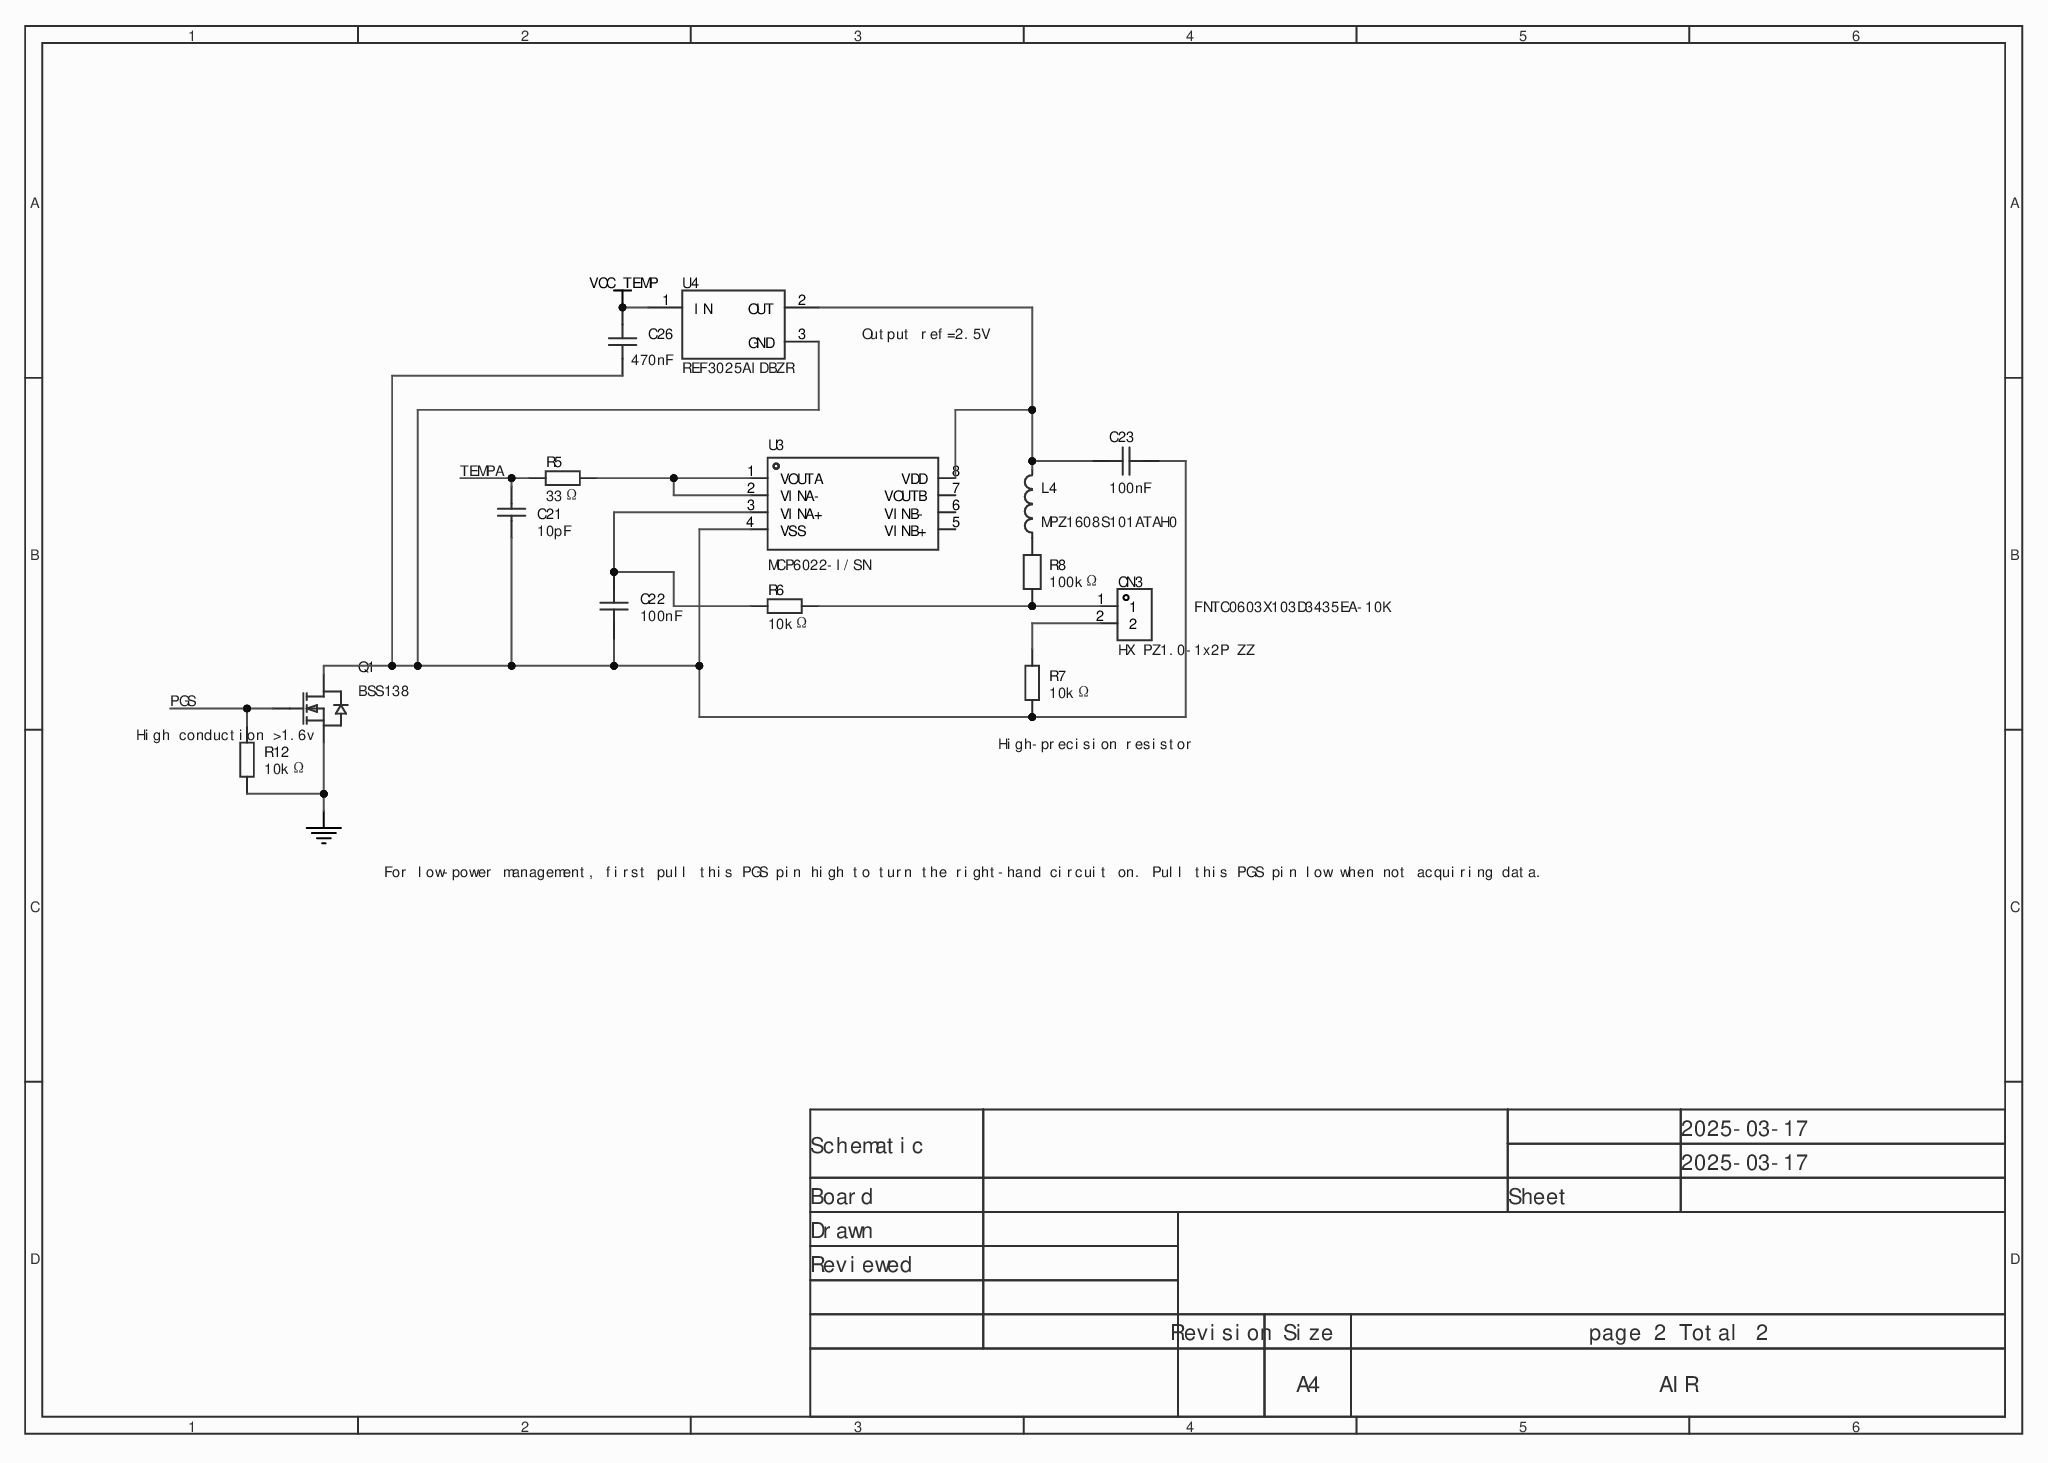
[diagram p0: MISC82703-4.schdoc]
# Altium project MISC82703-11.PrjPCB
2 sheets, 42 parts. Net scope: global (net labels, ports and power ports of the same name join across sheets).
Board file: MISC82703.PcbDoc
Sheets:
  MISC82703-4.schdoc
  MISC82703-2.schdoc

## Sheet MISC82703-4.schdoc
size 307 x 218 mm; Version: V1.0; @Project Name: MISC82703; @Page Count: 2; @Update Date: 2025-03-17; @Create Date: 2025-03-17; @Schematic Name: MISC82703; @Page No: 2; @Create Time: 21:29:07; @Update Time: 21:29:09; @Board Name: MISC82703

### Parts
C21  10pF  [C0402]
C22  100nF  [C0402]
C23  100nF  [C0402]
C26  470nF  [C0402]
CN3  HX PZ1.0-1x2P ZZ  [HDR-TH_2P-P1.00-V-M]
L4  MPZ1608S101ATAH0  [L0603]
Q1  BSS138  [SOT-23-3_L3.0-W1.7-P0.95-LS2.9-BR]
R5  33Ω  [R0402]
R6  10kΩ  [R0402]
R7  10kΩ  [R0402]
R8  100kΩ  [R0402]
R12  10kΩ  [R0402]
U3  MCP6022-I/SN  [SOIC-8_L4.9-W3.9-P1.27-LS6.0-BL]
U4  REF3025AIDBZR  [SOT-23-3_L2.9-W1.6-P1.90-LS2.8-BR]

### Nets
GND: Q1.2(S) R12.1
VCC_TEMP: C26.2 U4.1(IN)  [project net TL_VDD3]
PGS: Q1.1(G) R12.2
TEMPA: C21.2 R5.1
NetC21_1: C21.1 C22.1 C23.2 C26.1 Q1.3(D) R7.1 U3.4(VSS) U4.3(GND)
NetC22_2: C22.2 R6.2 U3.3(VINA+)
NetC23_1: C23.1 L4.2 U3.8(VDD) U4.2(OUT)
NetCN3_1: CN3.1 R6.1 R8.1
NetCN3_2: CN3.2 R7.2
NetL4_1: L4.1 R8.2
NetR5_2: R5.2 U3.1(VOUTA) U3.2(VINA-)

Not connected (* = marked no-connect by the designer): U3 5(VINB+)* 6(VINB-)* 7(VOUTB)*

### Notes on the sheet
- Output ref=2.5V
- FNTC0603X103D3435EA-10K
- High conduction >1.6v
- (near R7) High-precision resistor
- For low-power management, first pull this PGS pin high to turn the right-hand circuit on. Pull this PGS pin low when not acquiring data.
- 1
- 2
- 3
- 4
- 5
- 6
- A
- B
- C
- Schematic
- 2025-03-17
- Board
- Drawn
- Sheet
- D
- Reviewed
- Revision
- Size
- page 2 Total 2
- A4
- AIR

### Library data of the parts
C21 = CC0402JRNPO9BN100: Manufacturer: YAGEO(国巨); Add into BOM: yes; Tolerance: ±5%; Voltage Rated: 50V; Temperature Coefficient: NP0; Symbol: CC0402JRNPO9BN100; Device: CC0402JRNPO9BN100; LCSC Part Name: 10pF ±5% 50V; Supplier Part: C106199; Manufacturer Part: CC0402JRNPO9BN100; Supplier Footprint: 0402; JLCPCB Part Class: Extended library; Datasheet: https://atta.szlcsc.com/upload/public/pdf/source/20181008/C309499_21CC21451B82C39E3D92150FD6B30293.pdf; Supplier: LCSC; Convert to PCB: yes; Value: 10pF
C22 C23 = GRM155R71H104KE14D: Manufacturer: muRata(村田); Add into BOM: yes; Tolerance: ±10%; Voltage Rated: 50V; Temperature Coefficient: X7R; Symbol: GRM155R71H104KE14D; Device: GRM155R71H104KE14D; LCSC Part Name: 100nF ±10% 50V; Supplier Part: C77020; Manufacturer Part: GRM155R71H104KE14D; Supplier Footprint: 0402; JLCPCB Part Class: Extended library; Datasheet: https://atta.szlcsc.com/upload/public/pdf/source/20180326/C77020_39BD49C951FF1AF0DB1F1FAC5AC1E401.pdf; Supplier: LCSC; Convert to PCB: yes; Value: 100nF
C26 = CGA0402X7R474K100GT: Manufacturer: HRE(芯声); Add into BOM: yes; Tolerance: ±10%; Voltage Rating: 10V; Temperature Coefficient: X7R; Symbol: CGA0402X7R474K100GT; Device: CGA0402X7R474K100GT; LCSC Part Name: 470nF ±10% 10V; Supplier Part: C36911354; Manufacturer Part: CGA0402X7R474K100GT; Supplier Footprint: 0402; JLCPCB Part Class: Extended library; Datasheet: https://atta.szlcsc.com/upload/public/pdf/source/20240730/15E240B916CFB7780FDE6BEDB418139D.pdf; Supplier: LCSC; Convert to PCB: yes; Value: 470nF
CN3 = HX PZ1.0-1x2P ZZ: Manufacturer: hanxia(韩下); Add into BOM: yes; Pin Structure: 1x2P; Pitch: 1mm; Circluar Pins/Square Pins: Square pin; Current Rating: 750mA; Symbol: HX PZ1.0-1X2P ZZ; Device: HX PZ1.0-1x2P ZZ; LCSC Part Name: 1x2P 间距:1mm 方针 直插; Supplier Part: C22438170; Manufacturer Part: HX PZ1.0-1x2P ZZ; Supplier Footprint: 插件,P=1mm; Datasheet: https://atta.szlcsc.com/upload/public/pdf/source/20240522/59E077311630E4900351916CE6BE2E74.pdf; Supplier: LCSC; Convert to PCB: yes; Row Spacing: -; Mounting Type: Through hole; Number of Rows: Single row; Number of Pins: 2P; Voltage Rating (Max): -; Length of Mating Pin: 2mm; Insulation Height: 1mm; Length of End Connection Pin: 2mm; Contact Material: Phosphor bronze; Contact Plating: Gold; Operating Temperature: -40℃~+105℃; Color: Black
L4 = MPZ1608S101ATAH0: Manufacturer: TDK; Add into BOM: yes; Impedance @ Frequency: 100Ω@100MHz; Tolerance: ±25%; DC Resistance: 30mΩ; Current Rating: 3A; Circuits: 1; Symbol: MPZ1608S101ATAH0; Device: MPZ1608S101ATAH0; LCSC Part Name: 单路 0603磁珠 阻抗100Ω@100MHz; Supplier Part: C107332; Manufacturer Part: MPZ1608S101ATAH0; Supplier Footprint: 0603; JLCPCB Part Class: Extended library; Datasheet: https://atta.szlcsc.com/upload/public/pdf/source/20170420/1492670791787.pdf; Supplier: LCSC; Convert to PCB: yes
Q1 = BSS138: Manufacturer: AnBon(安邦); Symbol: BSS138_C193019; Add into BOM: yes; Type: 1 N-channel; Drain Source Voltage (Vdss): 50V; Continuous Drain Current (Id): 220mA; Drain Source On Resistance (RDS(on)@Vgs,Id): 3Ω@500mA,10V; Power Dissipation (Pd): 350mW; Gate Threshold Voltage (Vgs(th)@Id): 1.6V@250uA; Input Capacitance (Ciss@Vds): 27pF@25V; Device: BSS138; LCSC Part Name: 1个N沟道 耐压:50V 电流:220mA; Supplier Part: C193019; Manufacturer Part: BSS138; Supplier Footprint: SOT-23; Datasheet: https://atta.szlcsc.com/upload/public/pdf/source/20211210/347DFC394D39E807114CACD42CDBB225.pdf; Supplier: LCSC; Convert to PCB: yes; Total Gate Charge (Qg@Vgs): -; Reverse Transfer Capacitance (Crss@Vds): -
R5 = RC0402FR-0733RL: Manufacturer: YAGEO(国巨); Add into BOM: yes; Tolerance: ±1%; Power(Watts): 62.5mW; Overload Voltage (Max): 50V; Temperature Coefficient: ±100ppm/℃; Symbol: RC0402FR-0733RL; Device: RC0402FR-0733RL; LCSC Part Name: 厚膜电阻 33Ω ±1% 62.5mW; Supplier Part: C138002; Manufacturer Part: RC0402FR-0733RL; Supplier Footprint: 0402; JLCPCB Part Class: Extended library; Datasheet: https://atta.szlcsc.com/upload/public/pdf/source/20181009/C309620_DA5935B6E1D48212CB7A533FE518B3C2.pdf; Supplier: LCSC; Convert to PCB: yes; Type: Thick film resistor; Value: 33Ω; Operating Temperature Range: -55℃~+155℃
R6 R7 = RT0402BRD0710KL: Manufacturer: YAGEO(国巨); Add into BOM: yes; Tolerance: ±0.1%; Power(Watts): 62.5mW; Overload Voltage (Max): 50V; Temperature Coefficient: ±25ppm/℃; Symbol: RT0402BRD0710KL; Device: RT0402BRD0710KL; LCSC Part Name: 薄膜电阻 10kΩ ±0.1% 62.5mW; Supplier Part: C190095; Manufacturer Part: RT0402BRD0710KL; Supplier Footprint: 0402; Datasheet: https://atta.szlcsc.com/upload/public/pdf/source/20181009/C309664_C7CEF5A7F4D0541F96EF5E54D941D229.pdf; Supplier: LCSC; Convert to PCB: yes; Type: Thin film resistor; Value: 10kΩ; Operating Temperature Range: -55℃~+155℃
R8 = RT0402BRD07100KL: Manufacturer: YAGEO(国巨); Add into BOM: yes; Tolerance: ±0.1%; Power(Watts): 62.5mW; Overload Voltage (Max): 50V; Temperature Coefficient: ±25ppm/℃; Symbol: RT0402BRD07100KL; Device: RT0402BRD07100KL; LCSC Part Name: 薄膜电阻 100kΩ ±0.1% 62.5mW; Supplier Part: C852472; Manufacturer Part: RT0402BRD07100KL; Supplier Footprint: 0402; Datasheet: https://atta.szlcsc.com/upload/public/pdf/source/20210326/C852472_6283D268A9C33EA67274729CC55E28B1.pdf; Supplier: LCSC; Convert to PCB: yes; Type: Thin film resistor; Value: 100kΩ; Operating Temperature Range: -55℃~+155℃
R12 = 0402WGF1002TCE: Manufacturer: UNI-ROYAL(厚声); Add into BOM: yes; Tolerance: ±1%; Power(Watts): 62.5mW; Overload Voltage (Max): 50V; Temperature Coefficient: ±100ppm/℃; Symbol: 0402WGF1002TCE; Device: 0402WGF1002TCE; LCSC Part Name: 10kΩ ±1% 62.5mW 厚膜电阻; Supplier Part: C25744; Manufacturer Part: 0402WGF1002TCE; Supplier Footprint: 0402; JLCPCB Part Class: Basic library; Datasheet: https://atta.szlcsc.com/upload/public/pdf/source/20200306/C422600_1E6D84923E4A46A82E41ADD87F860B5C.pdf; Supplier: LCSC; Convert to PCB: yes; Type: Thick film resistor; Value: 10kΩ; Operating Temperature Range: -55℃~+155℃
U3 = MCP6022-I/SN: Manufacturer: MICROCHIP(美国微芯); Add into BOM: yes; Number of Circuits: Dual channel; Gain Bandwidth Product(GBP): 10MHz; Current - Input Bias(Ib): 1pA; Voltage - Input Offset(Vos): 500uV; Slew Rate(SR): 7V/us; Output Current: 30mA; Supply Current: 1mA; Symbol: MCP6022-I/SN; Device: MCP6022-I/SN; LCSC Part Name: MCP6022-I/SN; Supplier Part: C34047; Manufacturer Part: MCP6022-I/SN; Supplier Footprint: SOIC-8; JLCPCB Part Class: Extended library; Datasheet: https://atta.szlcsc.com/upload/public/pdf/source/20151020/1457707482040.pdf; Supplier: LCSC; Convert to PCB: yes; -3db Bandwidth: -; Output Type: -; Rail to Rail: -; Operating Temperature: -40℃~+85℃
U4 = REF3025AIDBZR: Manufacturer: TI(德州仪器); Add into BOM: yes; Output Type: Fixed; Input Voltage: 2.55V~5.5V; Output Voltage: 2.5V; Output Current: 25mA; Tolerance: ±0.2%; Temperature Coefficient: 75ppm/℃; Reference Type: Series; Supply Current: 50uA; Noise - 1/10Hz to 10Hz: 28uVp-p; Noise - 10Hz to 10kHz: 80uVrms; Symbol: REF3025AIDBZR; Device: REF3025AIDBZR; LCSC Part Name: REF3025AIDBZR; Supplier Part: C11334; Manufacturer Part: REF3025AIDBZR; Supplier Footprint: SOT-23; JLCPCB Part Class: Extended library; Datasheet: https://www.ti.com/cn/lit/gpn/ref3020; Supplier: LCSC; Convert to PCB: yes; Operating Temperature: -40℃~+125℃@(Ta)

## Sheet MISC82703-2.schdoc
size 307 x 218 mm; Version: V1.0; @Page Count: 2; @Update Date: 2025-05-15; @Create Date: 2025-05-15; @Schematic Name: MISC82703; @Page No: 1; @Create Time: 16:13:57; @Update Time: 16:13:59
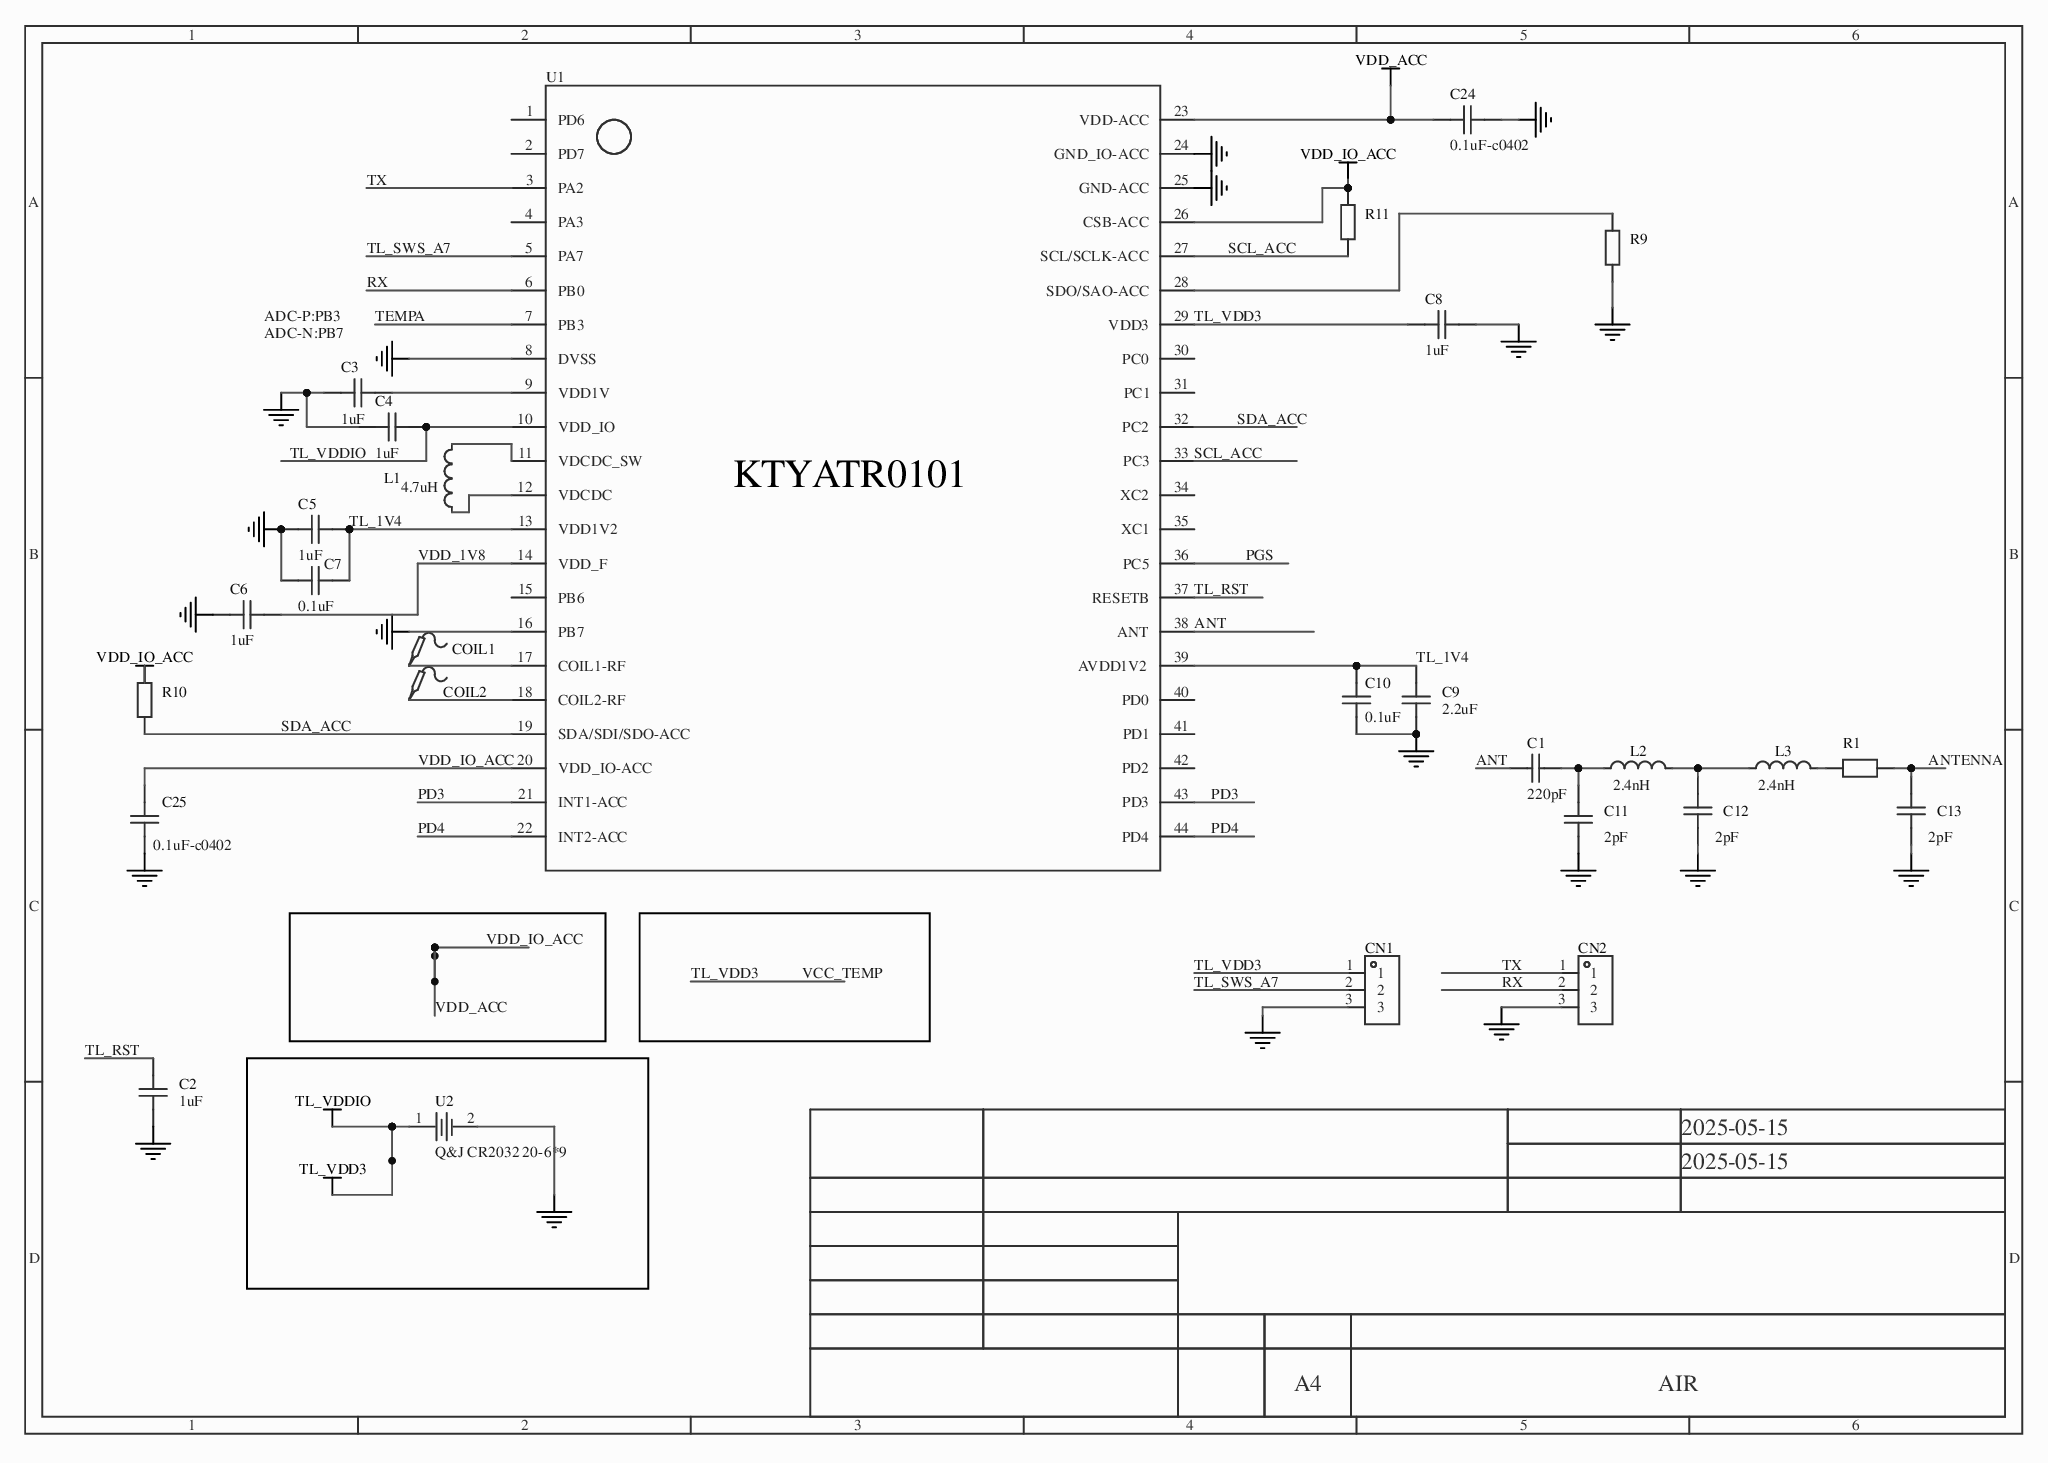
[diagram p1: MISC82703-2.schdoc]

### Parts
C1  220pF  [C0402]
C2  1uF  [C0402]
C3  1uF  [C0402]
C4  1uF  [C0402]
C5  1uF  [C0402]
C6  1uF  [C0402]
C7  0.1uF  [C0603]
C8  1uF  [C0402]
C9  2.2uF  [C0402]
C10  0.1uF  [C0402]
C11  2pF  [C0402]
C12  2pF  [C0402]
C13  2pF  [C0402]
C24  0.1uF-c0402  [C0402]
C25  0.1uF-c0402  [C0402]
CN1  (no value)  [HDR-TH_3P-P1.27-V-M-A]
CN2  (no value)  [HDR-TH_3P-P1.27-V-M-A]
COIL1  (no value)  [Test-Point-0.5mm]
COIL2  (no value)  [Test-Point-0.5mm]
L1  4.7uH  [IND-SMD_L1.8-W1.2]
L2  2.4nH  [L0402]
L3  2.4nH  [L0402]
R1  (no value)  [R0402]
R9  (no value)  [R0402]
R10  (no value)  [R0402]
R11  (no value)  [R0402]
U1  (no value)  [KTYATR0101]
U2  Q&J CR2032 20-6*9  [BAT-TH_CR2032]

### Nets
GND: C2.1 C3.1 C4.1 C5.1 C6.1 C7.1 C8.2 C9.1 C10.1 C11.1 C12.1 C13.1 C24.2 C25.2 CN1.3 CN2.3 R9.1 U1.8(DVSS) U1.16(PB7) U1.24(GND_IO-ACC) U1.25(GND-ACC) U2.2(-)
TL_VDD3: C4.2 C8.1 CN1.1 U1.10(VDD_IO) U1.29(VDD3) U2.1(+)  [also labelled TL_VDDIO, VCC_TEMP]
VDD_ACC: C24.1 C25.1 R10.2 R11.2 U1.20(VDD_IO-ACC) U1.23(VDD-ACC) U1.26(CSB-ACC)  [also labelled VDD_IO_ACC]
ANT: C1.1 U1.38(ANT)
ANTENNA: C13.2 R1.2
PD3: U1.21(INT1-ACC) U1.43(PD3)
PD4: U1.22(INT2-ACC) U1.44(PD4)
PGS: U1.36(PC5)
RX: CN2.2 U1.6(PB0)
SCL_ACC: R11.1 U1.27(SCL/SCLK-ACC) U1.33(PC3)
SDA_ACC: R10.1 U1.19(SDA/SDI/SDO-ACC) U1.32(PC2)
TEMPA: U1.7(PB3)
TL_1V4: C5.2 C7.2 C9.2 C10.2 U1.13(VDD1V2) U1.39(AVDD1V2)
TL_RST: C2.2 U1.37(RESETB)
TL_SWS_A7: CN1.2 U1.5(PA7)
TX: CN2.1 U1.3(PA2)
VDD_1V8: C6.2 U1.14(VDD_F)
NetC1_2: C1.2 C11.2 L2.1
NetC3_2: C3.2 U1.9(VDD1V)
NetC12_2: C12.2 L2.2 L3.1
NetCOIL1_1: COIL1.1 U1.17(COIL1-RF)
NetCOIL2_1: COIL2.1 U1.18(COIL2-RF)
NetL1_1: L1.1 U1.12(VDCDC)
NetL1_2: L1.2 U1.11(VDCDC_SW)
NetL3_2: L3.2 R1.1
NetR9_2: R9.2 U1.28(SDO/SAO-ACC)

Not connected (* = marked no-connect by the designer): U1 1(PD6)* 2(PD7)* 4(PA3)* 15(PB6)* 30(PC0)* 31(PC1)* 34(XC2)* 35(XC1)* 40(PD0)* 41(PD1)* 42(PD2)*

### Notes on the sheet
- ADC-P:PB3
  ADC-N:PB7
- 1
- 2
- 3
- 4
- 5
- 6
- A
- B
- C
- 2025-05-15
- D
- A4
- AIR

### Library data of the parts
C1 = CC0402KRX7R9BB221: Add into BOM: yes; Voltage Rated: 50V; Temperature Coefficient: X7R; Symbol: CC0402KRX7R9BB221; Device: CC0402KRX7R9BB221; Supplier Part: C107025; Manufacturer Part: CC0402KRX7R9BB221; Supplier Footprint: 0402; Datasheet: https://atta.szlcsc.com/upload/public/pdf/source/20170914/C128857_1505359892143968080.pdf; Supplier: LCSC; Convert to PCB: yes; Value: 220pF
C2-C6 C8-C10 = CL05A105KA5NQNC: Add into BOM: yes; Voltage Rated: 25V; Temperature Coefficient: X5R; Symbol: CL05A105KA5NQNC; Device: CL05A105KA5NQNC; Manufacturer Part: CL05A105KA5NQNC; Supplier Footprint: 0402; Datasheet: https://atta.szlcsc.com/upload/public/pdf/source/20160218/1457707763339.pdf; Supplier: LCSC; Convert to PCB: yes
  C2-C6 C8: Supplier Part: C52923; Value: 1uF
  C9: Value: 2.2uF
  C10: Value: 0.1uF
C7 = CAP_0603: Symbol: CapAcitance; Convert to PCB: yes; Device: CAP_0603; Add into BOM: yes; Supplier Footprint: 0603; Value: 0.1uF
C11-C13 = CC0402CRNPO9BN2R0: Add into BOM: yes; Voltage Rated: 50V; Temperature Coefficient: NP0; Symbol: CC0402CRNPO9BN2R0; Device: CC0402CRNPO9BN2R0; LCSC Part Name: 2pF 50V; Supplier Part: C325454; Manufacturer Part: CC0402CRNPO9BN2R0; Supplier Footprint: 0402; Datasheet: https://atta.szlcsc.com/upload/public/pdf/source/20181031/C325454_B7E70B15058089EBAF4951E75AE2AD52.pdf; Supplier: LCSC; Convert to PCB: yes; Value: 2pF
C24 C25 = 0.1uF-c0402: Add into BOM: yes; Symbol: 0.1UF-C0402; Device: 0.1uF-c0402; LCSC Part Name: 0.1uF-c0402; Supplier Part: C9900008998; Manufacturer Part: 0.1uF-c0402; Supplier Footprint: C0402; Supplier: LCSC; Convert to PCB: yes
CN1 CN2 = 3Pin_1.27___: Add into BOM: yes; Supplier Part: C9900016311; Supplier: LCSC; Convert to PCB: yes
COIL1 COIL2 = Test-Point: Add into BOM: yes; Symbol: Test-Point; Device: Test-Point; Convert to PCB: yes
L1 = SLC1608F4R7KTT: Add into BOM: yes; Rated Current: 400mA; Symbol: SLC1608F4R7KTT; Device: SLC1608F4R7KTT; Supplier Part: C411909; Manufacturer Part: SLC1608F4R7KTT; Supplier Footprint: SMD,1.8x1.2mm; Datasheet: https://atta.szlcsc.com/upload/public/pdf/source/20190822/C411909_D8F21CE75389351171F329DA46ED7C51.pdf; Supplier: LCSC; Convert to PCB: yes; Value: 4.7uH; Saturation Current (Isat): -; Q @ Freq: -; Frequency - Self Resonant: -; Ratings: -
L2 L3 = LQG15HH2N4S02D: Add into BOM: yes; Rated Current: 300mA; Q @ Freq: 8@100MHz; Frequency - Self Resonant: 6GHz; Symbol: LQG15HH2N4S02D; Device: LQG15HH2N4S02D; LCSC Part Name: 2.4nH; Supplier Part: C602035; Manufacturer Part: LQG15HH2N4S02D; Supplier Footprint: 0402; Datasheet: https://atta.szlcsc.com/upload/public/pdf/source/20190906/C426650_6C25041EF2EDD01B4762A59734016F86.pdf; Supplier: LCSC; Convert to PCB: yes; Value: 2.4nH; Tolerance: -; Saturation Current (Isat): -; Ratings: -
R1 = SCR0402J0R: Add into BOM: yes; Power(Watts): 62.5mW; Overload Voltage (Max): 50V; Symbol: SCR0402J0R; Device: SCR0402J0R; Supplier Part: C3017451; Manufacturer Part: SCR0402J0R; Supplier Footprint: 0402; Datasheet: https://atta.szlcsc.com/upload/public/pdf/source/20220513/247AF9639BA21CF93567DC289CCC6A22.pdf; Supplier: LCSC; Convert to PCB: yes
R9-R11 = 0402WGF4701TCE: Add into BOM: yes; Power(Watts): 62.5mW; Overload Voltage (Max): 50V; Symbol: 0402WGF4701TCE; Device: 0402WGF4701TCE; Supplier Part: C25900; Manufacturer Part: 0402WGF4701TCE; Supplier Footprint: 0402; Datasheet: https://atta.szlcsc.com/upload/public/pdf/source/20200306/C422600_1E6D84923E4A46A82E41ADD87F860B5C.pdf; Supplier: LCSC; Convert to PCB: yes
U1 = KTYATR0101: Add into BOM: yes; Symbol: KTYATR0101; Device: KTYATR0101; Convert to PCB: yes
U2 = Q&J CR2032 20-6*9: Add into BOM: yes; voltage: 3V; capacity: 240mAh; Device: Q&J CR2032 20-6*9; Supplier Part: C70382; Manufacturer: Q&J; Manufacturer Part: Q&J CR2032 20-6*9; Supplier Footprint: -; Datasheet: https://atta.szlcsc.com/upload/public/pdf/source/20170428/1493376822625.pdf; Supplier: LCSC; Convert to PCB: yes; battery model: -; Type of electrolyte: -

## Nets that join several sheets
GND: MISC82703-4 (Q1.2 R12.1), MISC82703-2 (22 pins)
TL_VDD3: MISC82703-4 (C26.2 U4.1), MISC82703-2 (6 pins)
PGS: MISC82703-4 (Q1.1 R12.2), MISC82703-2 (U1.36)
TEMPA: MISC82703-4 (C21.2 R5.1), MISC82703-2 (U1.7)